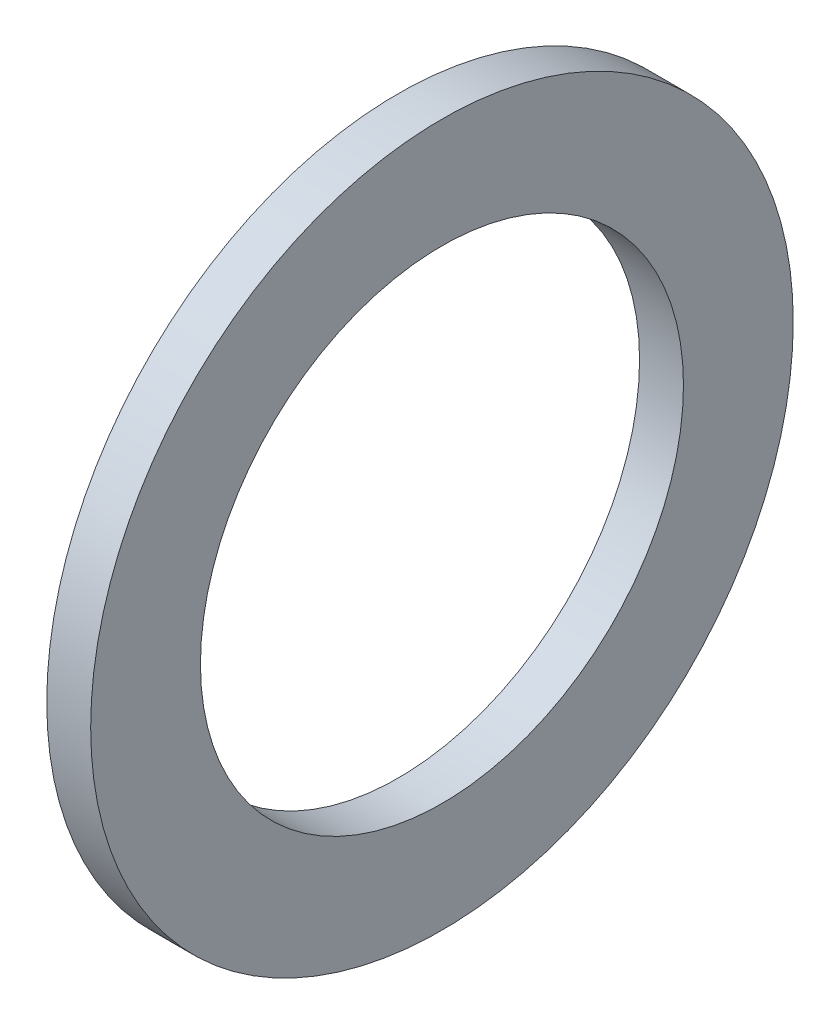
SolidWorks part; units mm, degrees
ref_plane "Front" through (0, 0, 0) normal (0, 0, 1) x (1, 0, 0)
ref_plane "Top" through (0, 0, 0) normal (0, 1, 0) x (1, 0, 0)
ref_plane "Right" through (0, 0, 0) normal (1, 0, 0) x (0, 0, -1)
sketch "Sketch1" plane through (0, 0, 0) normal (0, 0, 1) x (1, 0, 0)
  line L0 (0, 0) -> (-18.2441, 0) construction
  line L1 (0, 11) -> (2, 11)
  line L2 (0, 11) -> (0, 16)
  line L3 (0, 16) -> (2, 16)
  line L4 (2, 11) -> (2, 16)
  dimension "D1" = 2
  dimension "D2" = 5
  dimension "D3" = 11
revolve "Revolve1" add sketch "Sketch1" angle 360 about L0
